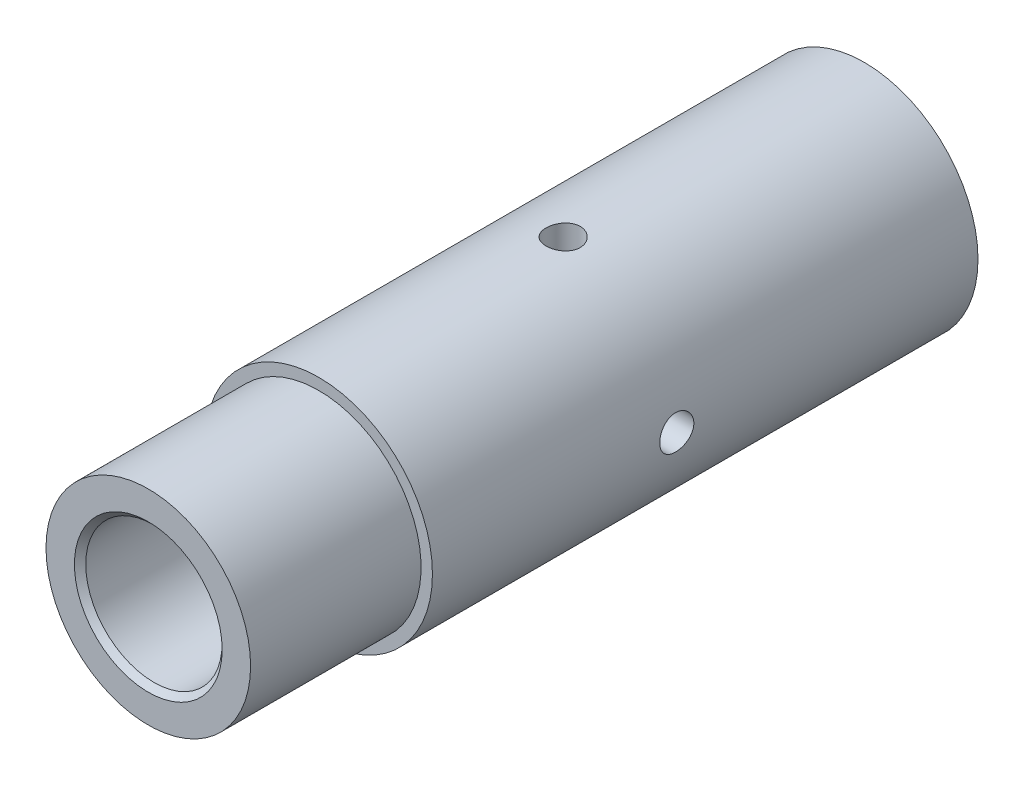
SolidWorks part; units mm, degrees
ref_plane "Front Plane" through (0, 0, 0) normal (0, 0, 1) x (1, 0, 0)
ref_plane "Top Plane" through (0, 0, 0) normal (0, 1, 0) x (1, 0, 0)
ref_plane "Right Plane" through (0, 0, 0) normal (1, 0, 0) x (0, 0, -1)
sketch "Sketch1" plane through (0, 0, 0) normal (0, 0, 1) x (1, 0, 0)
  circle A0 centre (0, 0) radius 9
  dimension "D1" = 18
extrude "Boss-Extrude1" add sketch "Sketch1" along normal blind 63
sketch "Sketch2" plane through (0, 0, 0) normal (0, 0, -1) x (-1, 0, 0)
  circle A0 centre (0, 0) radius 10
  dimension "D1" = 20
extrude "Boss-Extrude2" add sketch "Sketch2" against normal blind 48
sketch "Sketch3" plane through (0, 0, 0) normal (0, 0, -1) x (-1, 0, 0)
  circle A0 centre (0, 0) radius 6
  dimension "D1" = 12
extrude "Cut-Extrude1" cut sketch "Sketch3" against normal through all
sketch "Sketch4" plane through (0, 0, 0) normal (1, 0, 0) x (0, 0, -1)
  line L0 (0, 11) -> (0, -11) construction
  line L1 (-26.5, 14.4254) -> (-25, 14.4254)
  line L2 (-26.5, 14.4254) -> (-26.5, -13.2546)
  line L3 (-26.5, -13.2546) -> (-25, -13.2546)
  line L4 (-25, 14.4254) -> (-25, -13.2546)
  dimension "D1" = 27.68
  dimension "D2" = 1.5
  dimension "D3" = 26.5
revolve "Cut-Revolve1" cut sketch "Sketch4" angle 360 about L2
pattern_circular "CirPattern1" count 4 over 360 about axis through (0, 0, 48) along (0, 0, -1) of "Cut-Revolve1"
chamfer "Chamfer1" distance 0.5 angle 45 1 edges at (-6, 0, 63)
